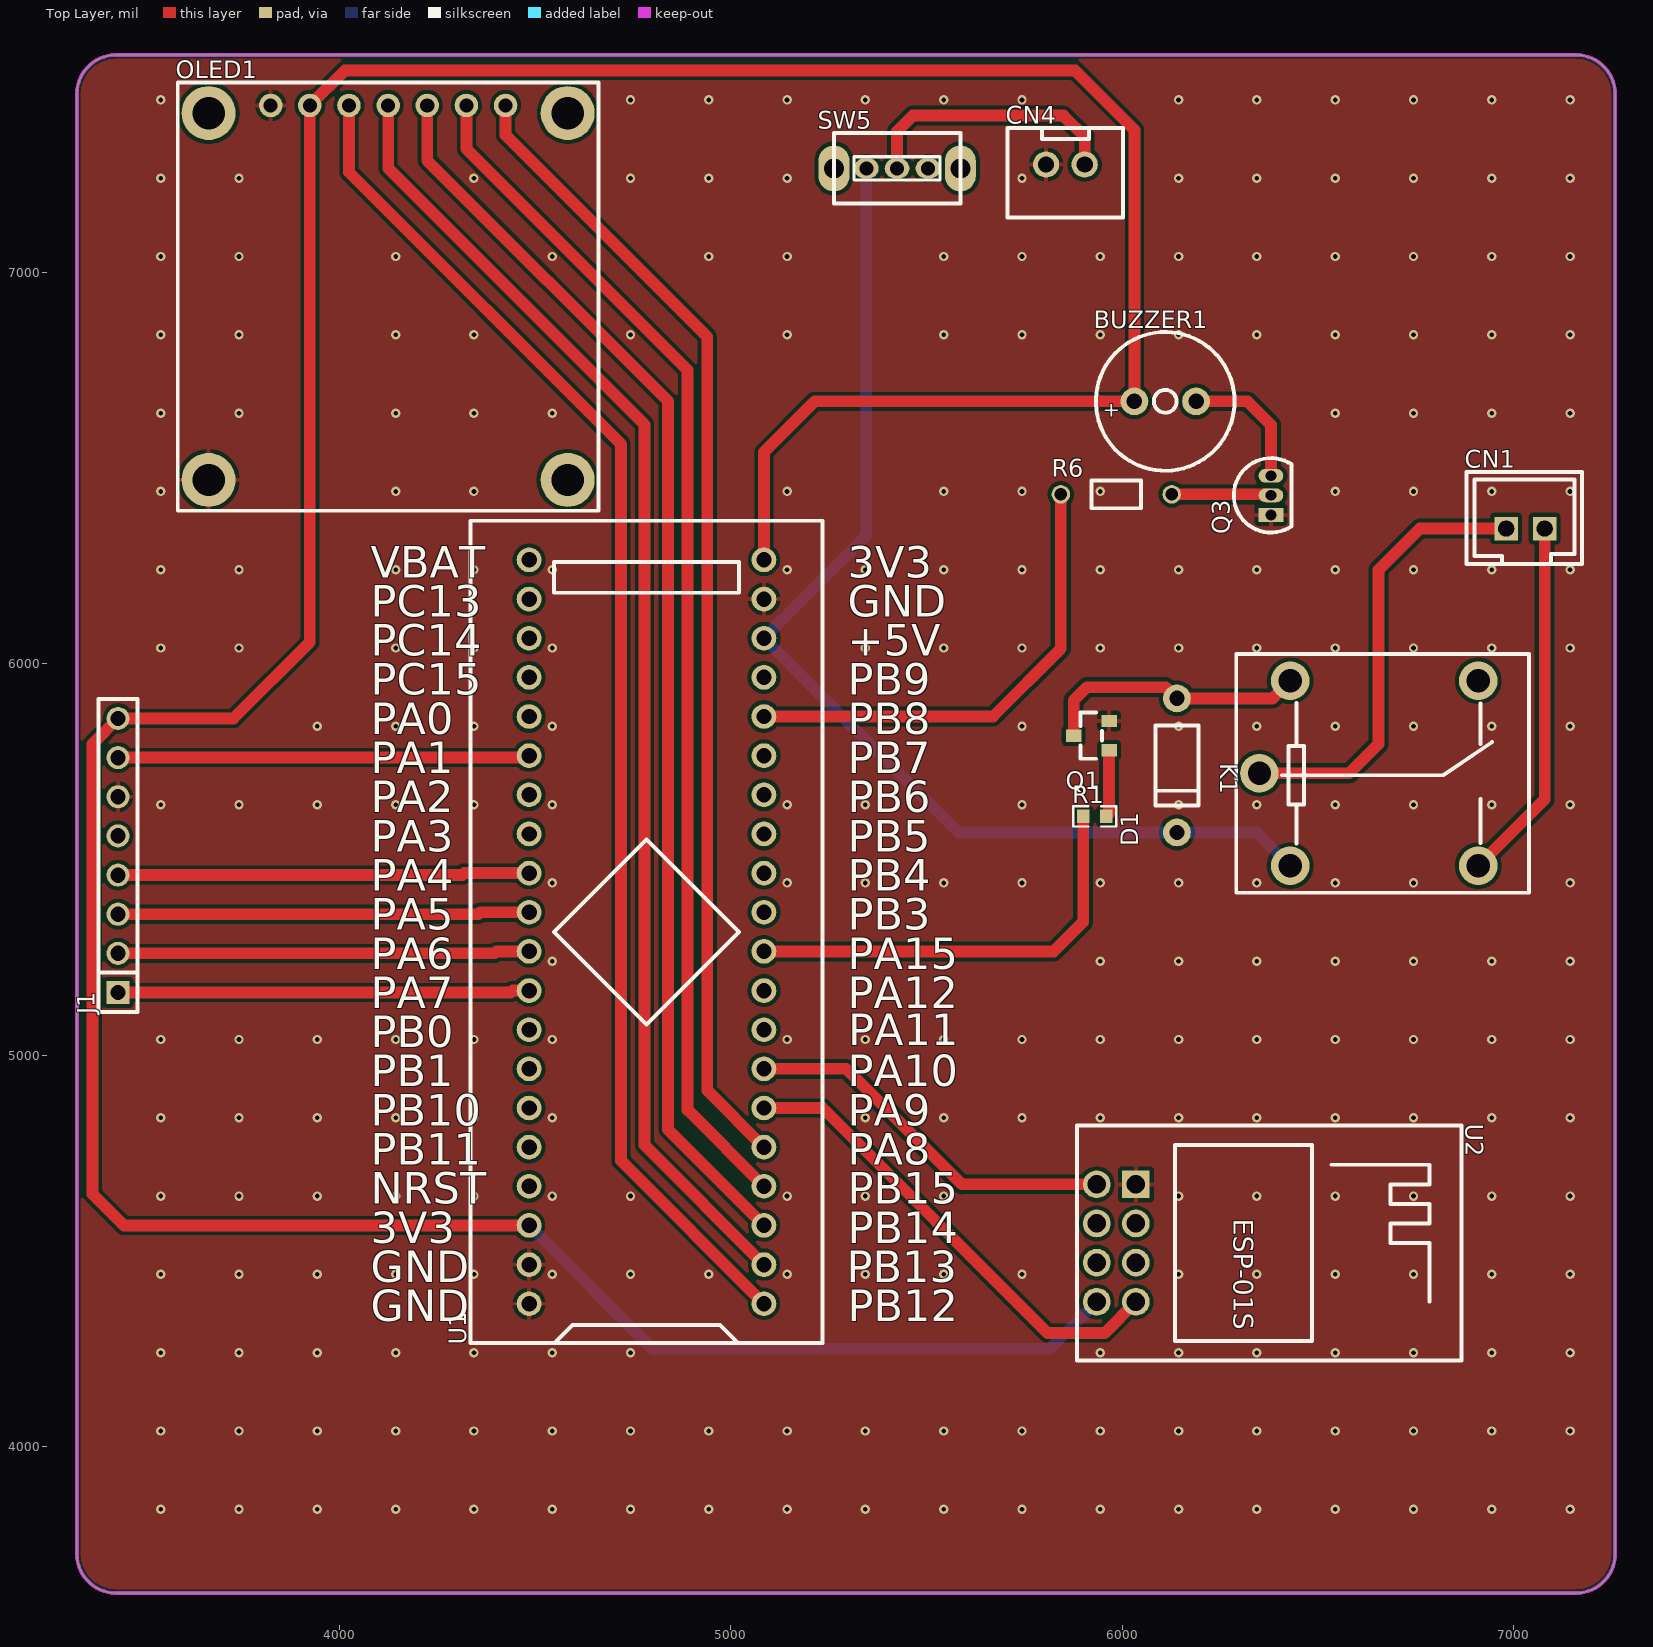
[diagram p0: Top Layer view]
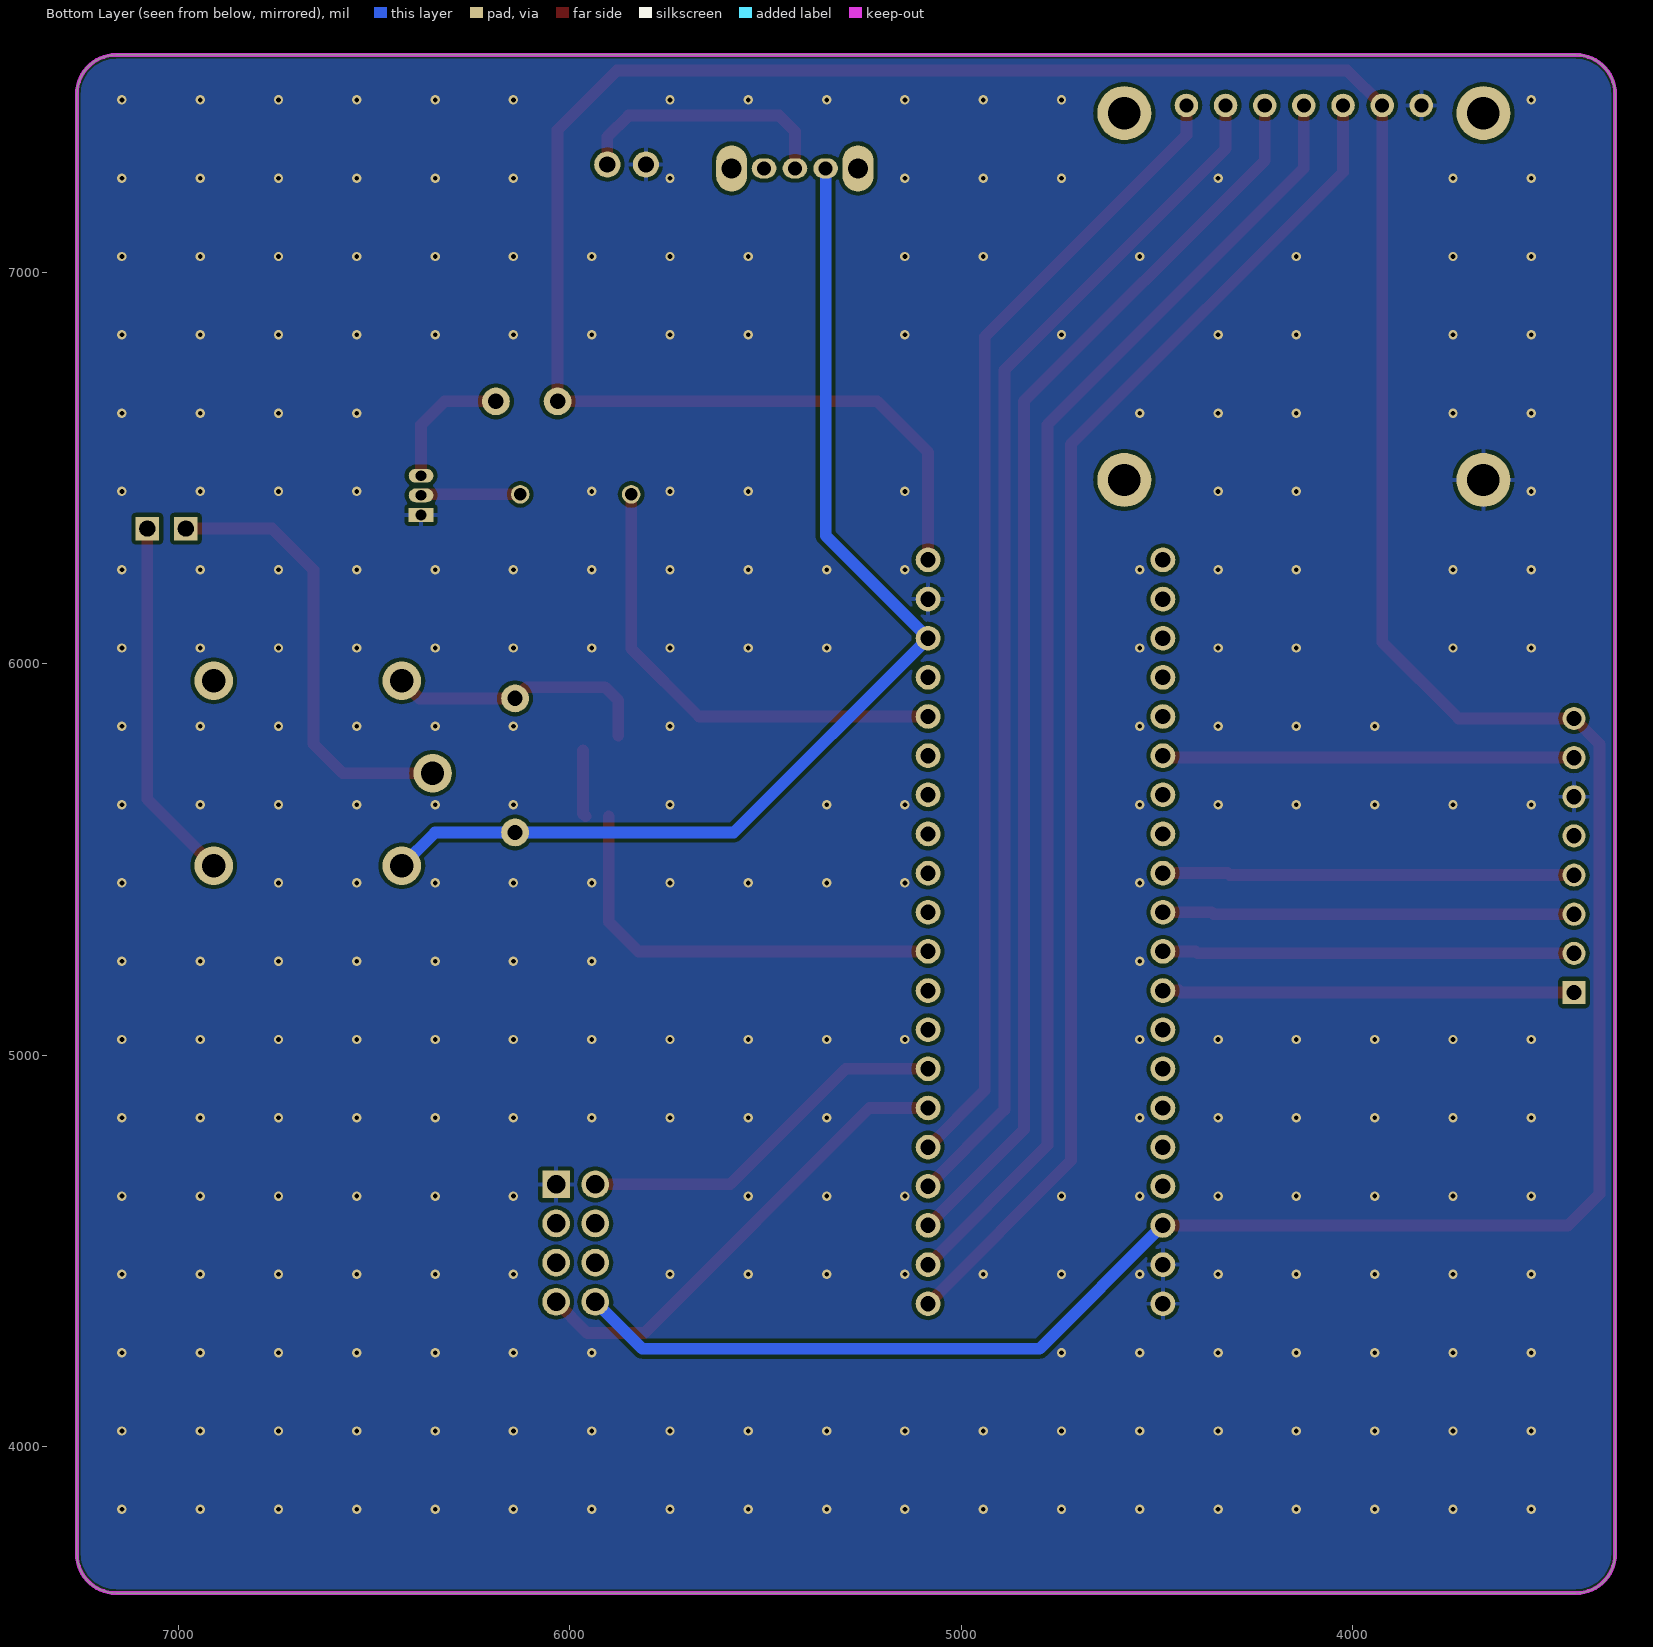
[diagram p1: Bottom Layer view, seen from below]
# Altium PCB MISC62443.pcbdoc
Units mil, origin at the board's own origin, x right, y up, seen from the top; angles counter-clockwise.
Board outline 3929.13 x 3929.13 mil, 2 copper layers (Top Layer, Bottom Layer), stack 62.206 mil thick; 14 components, 43 nets, 95 pads, 271 vias.

## Layer stack, top to bottom
Top Solder Mask Layer: solder mask 0.394, Dk 3.3
Top Layer: signal copper 1.379
Dielectric1: surface 59.449, FR4, Dk 4.5
Bottom Layer: signal copper 1.378
Bottom Solder Mask Layer: solder mask 0.394, Dk 3.3

## Board outline
3430,7555 ccw(c3430,7455) 3330,7455 3330,3725.87 ccw(c3430,3725.87) 3430,3625.87 7159.13,3625.87 ccw(c7159.13,3725.87) 7259.13,3725.87 7259.13,7455 ccw(c7159.13,7455) 7159.13,7555

## Design rules (kind name [scope] priority, off if disabled: settings)
BoardOutlineClearance copperThickness2oz_1 [All] p2 off: genericclearance=7.99 ignorepadtopadclearanceinfootprint=FALSE except(0: Arc-SplitContinuation Track-SplitContinuation SMDPad-SplitContinuation THPad-SplitContinuation Via-SplitContinuation Fill-SplitContinuation Region-SplitContinuation Poly-SplitContinuation Text-SplitContinuation Hole-SplitContinuation; 5.98: Arc-CutoutEdge Track-CutoutEdge SMDPad-CutoutEdge THPad-CutoutEdge Via-CutoutEdge Text-CutoutEdge; 6.9: Hole-OutlineEdge Hole-CutoutEdge; 10: Poly-OutlineEdge Poly-CutoutEdge; 11.81: Arc-OutlineEdge Track-OutlineEdge SMDPad-OutlineEdge THPad-OutlineEdge Via-OutlineEdge Fill-OutlineEdge Region-OutlineEdge Text-OutlineEdge Fill-CutoutEdge Region-CutoutEdge)
BoardOutlineClearance Plane_innerPlane_1 [All] p4 off: genericclearance=4.02 ignorepadtopadclearanceinfootprint=FALSE except(0: Arc-SplitContinuation Track-SplitContinuation SMDPad-SplitContinuation THPad-SplitContinuation Via-SplitContinuation Fill-SplitContinuation Region-SplitContinuation Poly-SplitContinuation Text-SplitContinuation Hole-SplitContinuation; 5.98: Arc-CutoutEdge Track-CutoutEdge SMDPad-CutoutEdge THPad-CutoutEdge Via-CutoutEdge Text-CutoutEdge; 6.9: Hole-OutlineEdge Hole-CutoutEdge; 10: Poly-OutlineEdge Poly-CutoutEdge; 11.81: Arc-OutlineEdge Track-OutlineEdge SMDPad-OutlineEdge THPad-OutlineEdge Via-OutlineEdge Fill-OutlineEdge Region-OutlineEdge Text-OutlineEdge Fill-CutoutEdge Region-CutoutEdge)
BoardOutlineClearance Copper_copperRegion_1 [All] p6 off: genericclearance=4.02 ignorepadtopadclearanceinfootprint=FALSE except(0: Arc-SplitContinuation Track-SplitContinuation SMDPad-SplitContinuation THPad-SplitContinuation Via-SplitContinuation Fill-SplitContinuation Region-SplitContinuation Poly-SplitContinuation Text-SplitContinuation Hole-SplitContinuation; 5.98: Arc-CutoutEdge Track-CutoutEdge SMDPad-CutoutEdge THPad-CutoutEdge Via-CutoutEdge Text-CutoutEdge; 6.9: Hole-OutlineEdge Hole-CutoutEdge; 10: Poly-OutlineEdge Poly-CutoutEdge; 11.81: Arc-OutlineEdge Track-OutlineEdge SMDPad-OutlineEdge THPad-OutlineEdge Via-OutlineEdge Fill-OutlineEdge Region-OutlineEdge Text-OutlineEdge Fill-CutoutEdge Region-CutoutEdge)
BoardOutlineClearance copperThickness1oz_1 [All] p8: genericclearance=4.02 ignorepadtopadclearanceinfootprint=FALSE except(0: Arc-SplitContinuation Track-SplitContinuation SMDPad-SplitContinuation THPad-SplitContinuation Via-SplitContinuation Fill-SplitContinuation Region-SplitContinuation Poly-SplitContinuation Text-SplitContinuation Hole-SplitContinuation; 5.98: Arc-CutoutEdge Track-CutoutEdge SMDPad-CutoutEdge THPad-CutoutEdge Via-CutoutEdge Text-CutoutEdge; 6.9: Hole-OutlineEdge Hole-CutoutEdge; 10: Poly-OutlineEdge Poly-CutoutEdge; 11.81: Arc-OutlineEdge Track-OutlineEdge SMDPad-OutlineEdge THPad-OutlineEdge Via-OutlineEdge Fill-OutlineEdge Region-OutlineEdge Text-OutlineEdge Fill-CutoutEdge Region-CutoutEdge)
Clearance copperThickness2oz [All] p1 off: gap=7.99 ignorepadtopadclearanceinfootprint=FALSE except(5.98: SMDPad-Track SMDPad-SMDPad THPad-Track SMDPad-THPad THPad-THPad Track-Via SMDPad-Via THPad-Via Via-Via Fill-SMDPad Region-SMDPad Fill-THPad Region-THPad Fill-Via Region-Via Fill-Fill Fill-Region Region-Region Arc-Track Arc-SMDPad Arc-THPad Arc-Via Fill-Arc Region-Arc Arc-Arc Text-Track SMDPad-Text Text-THPad Text-Via Fill-Text Region-Text Arc-Text Text-Text; 6.9: Hole-Track Hole-SMDPad Hole-THPad Hole-Via Fill-Hole Region-Hole Hole-Arc Hole-Text; 10: Poly-Track Poly-SMDPad Poly-THPad Poly-Via Poly-Fill Poly-Region Poly-Poly Poly-Arc Poly-Text Poly-Hole; 11.81: Fill-Track Region-Track)
Clearance Plane_innerPlane [All] p3 off: gap=4.02 ignorepadtopadclearanceinfootprint=FALSE except(5.98: SMDPad-Track SMDPad-SMDPad THPad-Track SMDPad-THPad THPad-THPad Track-Via SMDPad-Via THPad-Via Via-Via Fill-SMDPad Region-SMDPad Fill-THPad Region-THPad Fill-Via Region-Via Fill-Fill Fill-Region Region-Region Arc-Track Arc-SMDPad Arc-THPad Arc-Via Fill-Arc Region-Arc Arc-Arc Text-Track SMDPad-Text Text-THPad Text-Via Fill-Text Region-Text Arc-Text Text-Text; 6.9: Hole-Track Hole-SMDPad Hole-THPad Hole-Via Fill-Hole Region-Hole Hole-Arc Hole-Text; 10: Poly-Track Poly-SMDPad Poly-THPad Poly-Via Poly-Fill Poly-Region Poly-Poly Poly-Arc Poly-Text Poly-Hole; 11.81: Fill-Track Region-Track)
Clearance Copper_copperRegion [All] p5 off: gap=4.02 ignorepadtopadclearanceinfootprint=FALSE except(5.98: SMDPad-Track SMDPad-SMDPad THPad-Track SMDPad-THPad THPad-THPad Track-Via SMDPad-Via THPad-Via Via-Via Fill-SMDPad Region-SMDPad Fill-THPad Region-THPad Fill-Via Region-Via Fill-Fill Fill-Region Region-Region Arc-Track Arc-SMDPad Arc-THPad Arc-Via Fill-Arc Region-Arc Arc-Arc Text-Track SMDPad-Text Text-THPad Text-Via Fill-Text Region-Text Arc-Text Text-Text; 6.9: Hole-Track Hole-SMDPad Hole-THPad Hole-Via Fill-Hole Region-Hole Hole-Arc Hole-Text; 10: Poly-Track Poly-SMDPad Poly-THPad Poly-Via Poly-Fill Poly-Region Poly-Poly Poly-Arc Poly-Text Poly-Hole; 11.81: Fill-Track Region-Track)
Clearance copperThickness1oz [All] p7: gap=4.02 ignorepadtopadclearanceinfootprint=FALSE except(5.98: SMDPad-Track SMDPad-SMDPad THPad-Track SMDPad-THPad THPad-THPad Track-Via SMDPad-Via THPad-Via Via-Via Fill-SMDPad Region-SMDPad Fill-THPad Region-THPad Fill-Via Region-Via Fill-Fill Fill-Region Region-Region Arc-Track Arc-SMDPad Arc-THPad Arc-Via Fill-Arc Region-Arc Arc-Arc Text-Track SMDPad-Text Text-THPad Text-Via Fill-Text Region-Text Arc-Text Text-Text; 6.9: Hole-Track Hole-SMDPad Hole-THPad Hole-Via Fill-Hole Region-Hole Hole-Arc Hole-Text; 10: Poly-Track Poly-SMDPad Poly-THPad Poly-Via Poly-Fill Poly-Region Poly-Poly Poly-Arc Poly-Text Poly-Hole; 11.81: Fill-Track Region-Track)
DiffPairsRouting differentialPair [All] p1: maxlimit=6 minlimit=6 mostfreqgap=6 toplayer_minwidth=5 toplayer_prefwidth=10 toplayer_maxwidth=100 toplayer_mingap=6 toplayer_prefgap=6 toplayer_maxgap=6 bottomlayer_minwidth=5 bottomlayer_prefwidth=10 bottomlayer_maxwidth=100 bottomlayer_mingap=6 bottomlayer_prefgap=6 bottomlayer_maxgap=6 maxuncoupledlength=10
HoleToHoleClearance otherClearance [All] p1: gap=11.81 allowstackedmicrovias=TRUE
Length netLength [All] p1: minlimit=0 maxlimit=0
PasteMaskExpansion pasteMaskExpansion [All] p1: expansion=0
PlaneConnect innerPlane [All] p1: planeconnectstyle=Relief reliefexpansion=20 reliefentries=4 reliefconductorwidth=10 reliefairgap=10
PolygonConnect copperRegion [All] p1: connectstyle=Relief reliefconductorwidth=10 reliefentries=4 polygonreliefangle="90 Angle" airgapwidth=10 via.connectstyle=Relief via.reliefconductorwidth=10 via.reliefentries=4 via.polygonreliefangle="90 Angle" via.airgapwidth=10
RoutingVias viaSize [All] p1: holewidth=12.01 width=24.02 viastyle="Through Hole" minholewidth=11.81 minwidth=19.68 maxholewidth=248.03 maxwidth=393.7
SolderMaskExpansion solderMaskExpansion [IsVia] p1: expansion=-1000 istentingtop=TRUE
SolderMaskExpansion solderMaskExpansion [All] p2: expansion=2 istentingtop=FALSE
Width copperThickness2oz_2 [All] p1 off: maxlimit=100 minlimit=8 preferedwidth=10
Width copperThickness1oz_2 [All] p2: maxlimit=100 minlimit=5 preferedwidth=10

## Components (designator, comment, footprint, x,y, rotation, side; value= is the part's Value field where it differs from the comment)
BUZZER1 "2.7kHz" BUZ-TH_BD9.0-P4.00-D0.6-FD 6110,6670 r0 top
CN1 "XH2.54-2PIN-straight pin" CONN-TH_XH2.54-2P 7030,6345 r0 top
CN4 "XH2.54*2P_through-hole" CONN-TH_2P-P2.50-XH2.54-2P 5855,7275 r0 top
D1 "" DO_1N4007 6140,5740 r90 top
J1 "" HDR-TH_8P-P2.54-V-M 3435,5510 r90 top
K1 "HT3F-5VDC-SHG" RELAY-TH_HT3F-DCXX-X-X 6630,5720 r0 top
OLED1 "" 0.96OLED 4125,7485 r0 top
Q1 "" S8050_SOT-23 5921.34,5816.07 r0 top
Q3 "" S8050_TO_92 6380,6430 r90 top
R1 "1K" R0603 5930,5610 r0 top
R6 "1K" Res_1/8W 5985,6430 r0 top
SW5 "" 拨动开关 5420,7265 r0 top
U1 "LCKFB-DKX-STM32F103C8T6" CONN-TH_L53.3-W22.9_STM32F103C8T6-CARD 4785,5315 r90 top
U2 "ESP-01S" WIFIM-TH_ESP-01S 5985,4520 r270 top

## Footprints (in the part's own frame and the unit in brackets; to place one, negate y for a bottom-side part, rotate by r counter-clockwise, add the part's x,y. Pads: shape width x height; smd on the part's side, far side on the other; paste and mask are expansions set on the pad)
0.96OLED [mm]
  round 3.5 hole 2.1: 0(-11.65,-2) 1(-11.65,-25.8) 8(11.65,-2) 9(11.65,-25.8)
  round 1.524 hole 0.914: 1(-7.62,-1.5) 2(-5.08,-1.5) 3(-2.54,-1.5) 4(0,-1.5) 5(2.54,-1.5) 6(5.08,-1.5) 7(7.62,-1.5)
  silkscreen extent -13.65,-27.8 13.65,0
BUZ-TH_BD9.0-P4.00-D0.6-FD [mm]
  round 1.8 hole 1: 1(-2,0) 2(2,0)
  silkscreen extent -4.5,-4.5 4.5,4.5
CONN-TH_2P-P2.50-XH2.54-2P [mm]
  round 1.7 hole 1.05 paste+0 mask+0.05: 1(1.25,0) 2(-1.25,0)
  silkscreen extent -3.75,-3.42 3.75,2.37
CONN-TH_L53.3-W22.9_STM32F103C8T6-CARD [mm]
  round 1.6 hole 1: 1(-24.13,-7.62) 2(-21.59,-7.62) 3(-19.05,-7.62) 4(-16.51,-7.62) 5(-13.97,-7.62) 6(-11.43,-7.62) 7(-8.89,-7.62) 8(-6.35,-7.62) 9(-3.81,-7.62) 10(-1.27,-7.62) 11(1.27,-7.62) 12(3.81,-7.62) 13(6.35,-7.62) 14(8.89,-7.62) 15(11.43,-7.62) 16(13.97,-7.62) 17(16.51,-7.62) 18(19.05,-7.62) 19(21.59,-7.62) 20(24.13,-7.62) 21(24.13,7.62) 22(21.59,7.62) 23(19.05,7.62) 24(16.51,7.62) 25(13.97,7.62) 26(11.43,7.62) 27(8.89,7.62) 28(6.35,7.62) 29(3.81,7.62) 30(1.27,7.62) 31(-1.27,7.62) 32(-3.81,7.62) 33(-6.35,7.62) 34(-8.89,7.62) 35(-11.43,7.62) 36(-13.97,7.62) 37(-16.51,7.62) 38(-19.05,7.62) 39(-21.59,7.62) 40(-24.13,7.62)
  silkscreen extent -26.67,-11.43 26.67,11.43
CONN-TH_XH2.54-2P [mil]
  rect 60x60 hole 39.37 slot 41.34 at 0 deg paste+0 mask+1.97: 1(-49.22,0) 2(49.21,0)
  silkscreen extent -150,-90 145,145
DO_1N4007 [mm]
  round 1.8 hole 1 paste+0 mask+0.051: 1(-4.35,0) 2(4.35,0)
  silkscreen extent -2.6,-1.4 2.6,1.4
HDR-TH_8P-P2.54-V-M [mm]
  rect 1.5x1.5 hole 1: 1(-8.89,0)
  round 1.5 hole 1: 2(-6.35,0) 3(-3.81,0) 4(-1.27,0) 5(1.27,0) 6(3.81,0) 7(6.35,0) 8(8.89,0)
  silkscreen extent -10.16,-1.27 10.16,1.27
R0603 [mil]
  rect 31.75x34.02 smd paste-3937.01 mask+2: 1(-29.66,0) 2(29.66,0)
  silkscreen extent -55,-26 55,26
RELAY-TH_HT3F-DCXX-X-X [mm]
  round 2.5 hole 1.5: 1(-7.1,0) 2(-5.1,-6) 3(7.1,-6) 4(7.1,6) 5(-5.1,6)
  silkscreen extent -8.6,-7.75 10.4,7.75
Res_1/8W [mil]
  round 47.2 hole 31.5 paste+0 mask+2: 1(-141.7,2.48) 2(141.7,2.48)
  silkscreen extent -63,-33 63,38
S8050_SOT-23 [mm]
  rect 1x0.8 smd paste+0 mask+0.051: 1(1.15,-0.95) 2(1.15,0.95) 3(-1.15,0)
  silkscreen extent -0.7,-1.5 0.7,1.5
S8050_TO_92 [mil]
  rect 35.4x63 hole 27.6 paste+0 mask+2: 1(-50,0)
  oval 35.4x63 hole 27.6 paste+0 mask+2: 2(0,0) 3(50,0)
  silkscreen extent -95,-53 95,95
WIFIM-TH_ESP-01S [mm]
  rect 1.8x1.8 hole 1.2: 1(-3.81,1.27)
  round 1.8 hole 1.2: 2(-1.27,1.27) 3(1.27,1.27) 4(3.81,1.27) 5(3.81,-1.27) 6(1.27,-1.27) 7(-1.27,-1.27) 8(-3.81,-1.27)
  silkscreen extent -7.62,-2.54 7.62,22.4
拨动开关 [mil]
  oval 63x51.2 hole 35.4 paste+0 mask+2: 1(-73.4,0) 2(5,0) 3(84,0)
  oval 78.7x118.1 hole 51.2 paste+0 mask+2: 4(166.7,0) 5(-156.1,0)
  silkscreen extent -156,-90 167,90

## Via types
v1: diameter 24.02, hole 12, Top Layer to Bottom Layer, 271 vias

## Nets (pads, with @x,y where several pads share a name; then routed paths per layer and width w, separated by ;. In a path a pad name is that pad's centre, name@x,y a point inside that pad or via, vN(x,y) a via of type N, cw(c..) or ccw(c..) an arc to the next point about the centre after c; other vN are vias at no path point)
$1N416: U1.11
$1N421: U1.12
$1N426: U1.13
$1N431: U1.14
$1N436: U1.15
$1N446: U1.17
$1N490: U1.37
$1N495: U1.36
$1N500: U1.35
$1N505: U1.34
$1N510: U1.33
$1N535: U1.28
$1N595: U1.25
$1N602: U1.27
$1N607: U1.8
$1N1877: BUZZER1.2 Q3.3 | length 346.1
  Top Layer w30: BUZZER1.2 6320,6670 6380,6610 Q3.3
$1N2018: Q3.2 R6.2 | length 254.3
  Top Layer w30: R6.2 6377.52,6432.48 Q3.2
$1N5134: U1.22
$1N5154: CN1.1 K1.1 | length 1149.9
  Top Layer w30: K1.1 6580,5720 6655,5795 6655,6240 6760,6345 CN1.1
$1N5155: CN1.2 K1.3 | length 931.5
  Top Layer w30: K1.3 7079.22,5653.47 CN1.2
$1N5157: D1.2 K1.5 Q1.3 | length 687.7
  Top Layer w30: Q1.3 5876.06,5906.06 5910,5940 6111.26,5940 D1.2 6384.26,5911.26 K1.5
$1N5158: Q1.1 R1.2 | length 171.6
  Top Layer w30: R1.2 5966.62,5616.96 Q1.1
$1N5162: CN4.1 SW5.2 | length 684
  Top Layer w30: SW5.2 5425,7360 5465,7400 5850,7400 5904.22,7345.78 CN4.1
+5V: D1.1 K1.2 SW5.1 U1.18 | length 2893.3
  Bottom Layer w30: SW5.1 5346.6,6326.6 U1.18 5581.26,5568.74 D1.1 6344.26,5568.74 K1.2
BEEP: R6.1 U1.16 | length 1224.3
  Top Layer w30: U1.16 5670,5865 5843.3,6038.3 R6.1
GND: CN4.2 J1.6 OLED1.1 Q1.2 Q3.1 U1.19 U1.39 U1.40 U2.1
  other v1: 3544.1,3839.97 3744.1,3839.97 3944.1,3839.97 4144.1,3839.97 4344.1,3839.97 4544.1,3839.97 4744.1,3839.97 4944.1,3839.97 5144.1,3839.97 5344.1,3839.97 5544.1,3839.97 5744.1,3839.97 5944.1,3839.97 6144.1,3839.97 6344.1,3839.97 6544.1,3839.97 6744.1,3839.97 6944.1,3839.97 7144.1,3839.97 3544.1,4039.97 3744.1,4039.97 3944.1,4039.97 4144.1,4039.97 4344.1,4039.97 4544.1,4039.97 4744.1,4039.97 4944.1,4039.97 5144.1,4039.97 5344.1,4039.97 5544.1,4039.97 5744.1,4039.97 5944.1,4039.97 6144.1,4039.97 6344.1,4039.97 6544.1,4039.97 6744.1,4039.97 6944.1,4039.97 7144.1,4039.97 3544.1,4239.97 3744.1,4239.97 3944.1,4239.97 4144.1,4239.97 4344.1,4239.97 4544.1,4239.97 4744.1,4239.97 5944.1,4239.97 6144.1,4239.97 6344.1,4239.97 6544.1,4239.97 6744.1,4239.97 6944.1,4239.97 7144.1,4239.97 3544.1,4439.97 3744.1,4439.97 3944.1,4439.97 4144.1,4439.97 4344.1,4439.97 4544.1,4439.97 4744.1,4439.97 4944.1,4439.97 5144.1,4439.97 5344.1,4439.97 5544.1,4439.97 5744.1,4439.97 6144.1,4439.97 6344.1,4439.97 6544.1,4439.97 6744.1,4439.97 6944.1,4439.97 7144.1,4439.97 3544.1,4639.97 3744.1,4639.97 3944.1,4639.97 4144.1,4639.97 4344.1,4639.97 4544.1,4639.97 4744.1,4639.97 5144.1,4639.97 5344.1,4639.97 5544.1,4639.97 6144.1,4639.97 6344.1,4639.97 6544.1,4639.97 6744.1,4639.97 6944.1,4639.97 7144.1,4639.97 3544.1,4839.97 3744.1,4839.97 3944.1,4839.97 4144.1,4839.97 4344.1,4839.97 4544.1,4839.97 5344.1,4839.97 5544.1,4839.97 5744.1,4839.97 5944.1,4839.97 6144.1,4839.97 6344.1,4839.97 6544.1,4839.97 6744.1,4839.97 6944.1,4839.97 7144.1,4839.97 3544.1,5039.97 3744.1,5039.97 3944.1,5039.97 4144.1,5039.97 4344.1,5039.97 4544.1,5039.97 5144.1,5039.97 5344.1,5039.97 5544.1,5039.97 5744.1,5039.97 5944.1,5039.97 6144.1,5039.97 6344.1,5039.97 6544.1,5039.97 6744.1,5039.97 6944.1,5039.97 7144.1,5039.97 4544.1,5239.97 5944.1,5239.97 6144.1,5239.97 6344.1,5239.97 6544.1,5239.97 6744.1,5239.97 6944.1,5239.97 7144.1,5239.97 4544.1,5439.97 5144.1,5439.97 5344.1,5439.97 5544.1,5439.97 5744.1,5439.97 5944.1,5439.97 6144.1,5439.97 6344.1,5439.97 6544.1,5439.97 6744.1,5439.97 7144.1,5439.97 3544.1,5639.97 3744.1,5639.97 3944.1,5639.97 4144.1,5639.97 4344.1,5639.97 4544.1,5639.97 5144.1,5639.97 5344.1,5639.97 5744.1,5639.97 6144.1,5639.97 6344.1,5639.97 6544.1,5639.97 6744.1,5639.97 6944.1,5639.97 7144.1,5639.97 3944.1,5839.97 4144.1,5839.97 4344.1,5839.97 4544.1,5839.97 5744.1,5839.97 6144.1,5839.97 6344.1,5839.97 6544.1,5839.97 6744.1,5839.97 6944.1,5839.97 7144.1,5839.97 3544.1,6039.97 3744.1,6039.97 4144.1,6039.97 4344.1,6039.97 4544.1,6039.97 5344.1,6039.97 5544.1,6039.97 5744.1,6039.97 5944.1,6039.97 6144.1,6039.97 6344.1,6039.97 6544.1,6039.97 6744.1,6039.97 6944.1,6039.97 7144.1,6039.97 3544.1,6239.97 3744.1,6239.97 4144.1,6239.97 4344.1,6239.97 4544.1,6239.97 5144.1,6239.97 5344.1,6239.97 5544.1,6239.97 5744.1,6239.97 5944.1,6239.97 6144.1,6239.97 6344.1,6239.97 6544.1,6239.97 6744.1,6239.97 6944.1,6239.97 7144.1,6239.97 3544.1,6439.97 4144.1,6439.97 4344.1,6439.97 5144.1,6439.97 5544.1,6439.97 5744.1,6439.97 5944.1,6439.97 6544.1,6439.97 6744.1,6439.97 6944.1,6439.97 7144.1,6439.97 3544.1,6639.97 3744.1,6639.97 4144.1,6639.97 4344.1,6639.97 4544.1,6639.97 6544.1,6639.97 6744.1,6639.97 6944.1,6639.97 7144.1,6639.97 3544.1,6839.97 3744.1,6839.97 4144.1,6839.97 4344.1,6839.97 4744.1,6839.97 5144.1,6839.97 5544.1,6839.97 5744.1,6839.97 5944.1,6839.97 6144.1,6839.97 6344.1,6839.97 6544.1,6839.97 6744.1,6839.97 6944.1,6839.97 7144.1,6839.97 3544.1,7039.97 3744.1,7039.97 4144.1,7039.97 4544.1,7039.97 4944.1,7039.97 5144.1,7039.97 5544.1,7039.97 5744.1,7039.97 5944.1,7039.97 6144.1,7039.97 6344.1,7039.97 6544.1,7039.97 6744.1,7039.97 6944.1,7039.97 7144.1,7039.97 3544.1,7239.97 3744.1,7239.97 4344.1,7239.97 4744.1,7239.97 4944.1,7239.97 5144.1,7239.97 5744.1,7239.97 6144.1,7239.97 6344.1,7239.97 6544.1,7239.97 6744.1,7239.97 6944.1,7239.97 7144.1,7239.97 3544.1,7439.97 4744.1,7439.97 4944.1,7439.97 5144.1,7439.97 5344.1,7439.97 5544.1,7439.97 5744.1,7439.97 6144.1,7439.97 6344.1,7439.97 6544.1,7439.97 6744.1,7439.97 6944.1,7439.97 7144.1,7439.97
IN1: R1.1 U1.10 | length 1116.2
  Top Layer w30: U1.10 5825,5265 5900.34,5340.34 R1.1
IN2: U1.9
IN3: U1.24
IN4: U1.23
MFR_MISO: J1.4 U1.29 | length 1052.1
  Top Layer w30: J1.4 4314.24,5460 4319.24,5465 U1.29
MFR_MOSI: J1.3 U1.30 | length 1052.1
  Top Layer w30: J1.3 4355.66,5360 4360.66,5365 U1.30
MFR_RST: J1.7 U1.26 | length 1052.1
  Top Layer w30: J1.7 4480,5760 U1.26
MFR_SCK: J1.2 U1.31 | length 1052.1
  Top Layer w30: J1.2 4397.08,5260 4402.08,5265 U1.31
MFR_SDA: J1.1 U1.32 | length 1052.1
  Top Layer w30: J1.1 4438.5,5160 4443.5,5165 U1.32
OLED_CS: OLED1.7 U1.5 | length 2934.3
  Top Layer w30: OLED1.7 4425,7350 4940,6835 4940,4910 U1.5
OLED_D0: OLED1.3 U1.1 | length 3500
  Top Layer w30: OLED1.3 4025,7255 4720,6560 4720,4730 U1.1
OLED_D1: OLED1.4 U1.2 | length 3358.6
  Top Layer w30: OLED1.4 4125,7265 4780,6610 4780,4770 U1.2
OLED_DC: OLED1.6 U1.4 | length 3075.7
  Top Layer w30: OLED1.6 4325,7315 4890,6750 4890,4860 U1.4
OLED_RES: OLED1.5 U1.3 | length 3217.2
  Top Layer w30: OLED1.5 4225,7285 4840,6670 4840,4810 U1.3
UART1_RX: U1.7 U2.8 | length 972.2
  Top Layer w30: U1.7 5295,4965 5590,4670 U2.8
UATR1_TX: U1.6 U2.4 | length 1221.3
  Top Layer w30: U1.6 5235,4865 5810,4290 5955,4290 U2.4
VCC: BUZZER1.1 J1.8 OLED1.2 U1.20 U1.38 U2.5 | length 10136.6
  Top Layer w30: U1.38 3450,4565 3370,4645 3370,5795 J1.8 3730,5860 3925,6055 OLED1.2 4014.06,7515 5880,7515 6031.26,7363.74 BUZZER1.1 5215,6670 5085,6540 U1.20
  Bottom Layer w30: U1.38 4800,4250 5815,4250 U2.5
pads on no net: J1.5 K1.4 OLED1.0 OLED1.8 OLED1.9 SW5.3 SW5.4 SW5.5 U1.21 U2.2 U2.3 U2.6 U2.7

## Polygon pours and split planes (outlines as drawn)
GND on Top Layer (solid, remove dead copper, pour order 0): 3285,7570 3285,3590 7285,3590 7285,7570
GND on Bottom Layer (solid, remove dead copper, pour order 2): 3285,7575 3285,3600 7280,3600 7280,7575
GND on Bottom Layer (solid, remove dead copper, pour order 4): 3000,7815 3000,3000 7580,3000 7580,7815

## Keep-outs
Board Outline Layer:
  the board outline again, w10

## Silkscreen, mask and mechanical layers (free items; w line width, h text height)
Top Silkscreen Layer:
  text "VBAT" at 4080.95,6220 h80
  text "3V3" at 5299.16,6220 h80
  text "PC13" at 4080.95,6120 h80
  text "GND" at 5299.16,6120 h80
  text "PC14" at 4080.95,6020 h80
  text "+5V" at 5299.16,6020 h80
  text "PC15" at 4080.95,5920 h80
  text "PB9" at 5299.16,5920 h80
  text "PA0" at 4080.95,5820 h80
  text "PB8" at 5299.16,5820 h80
  text "PA1" at 4080.95,5720 h80
  text "PB7" at 5299.16,5720 h80
  text "PA2" at 4080.95,5620 h80
  text "PB6" at 5299.16,5620 h80
  text "PA3" at 4080.95,5520 h80
  text "PB5" at 5299.16,5520 h80
  text "PA4" at 4080.95,5420 h80
  text "PB4" at 5299.16,5420 h80
  text "PA5" at 4080.95,5320 h80
  text "PB3" at 5299.16,5320 h80
  text "PA6" at 4080.95,5220 h80
  text "PA15" at 5299.16,5220 h80
  text "PA7" at 4080.95,5120 h80
  text "PA12" at 5299.16,5120 h80
  text "PA11" at 5300.95,5025 h80
  text "PB0" at 4080.95,5020 h80
  text "PB1" at 4080.95,4920 h80
  text "PA10" at 5299.16,4920 h80
  text "PB10" at 4080.95,4820 h80
  text "PA9" at 5299.16,4820 h80
  text "PB11" at 4080.95,4720 h80
  text "PA8" at 5299.16,4720 h80
  text "NRST" at 4080.95,4620 h80
  text "PB15" at 5299.16,4620 h80
  text "3V3" at 4080.95,4520 h80
  text "PB14" at 5299.16,4520 h80
  text "GND" at 4080.95,4420 h80
  text "PB13" at 5295.95,4420 h80
  text "GND" at 4080.95,4320 h80
  text "PB12" at 5299.16,4320 h80